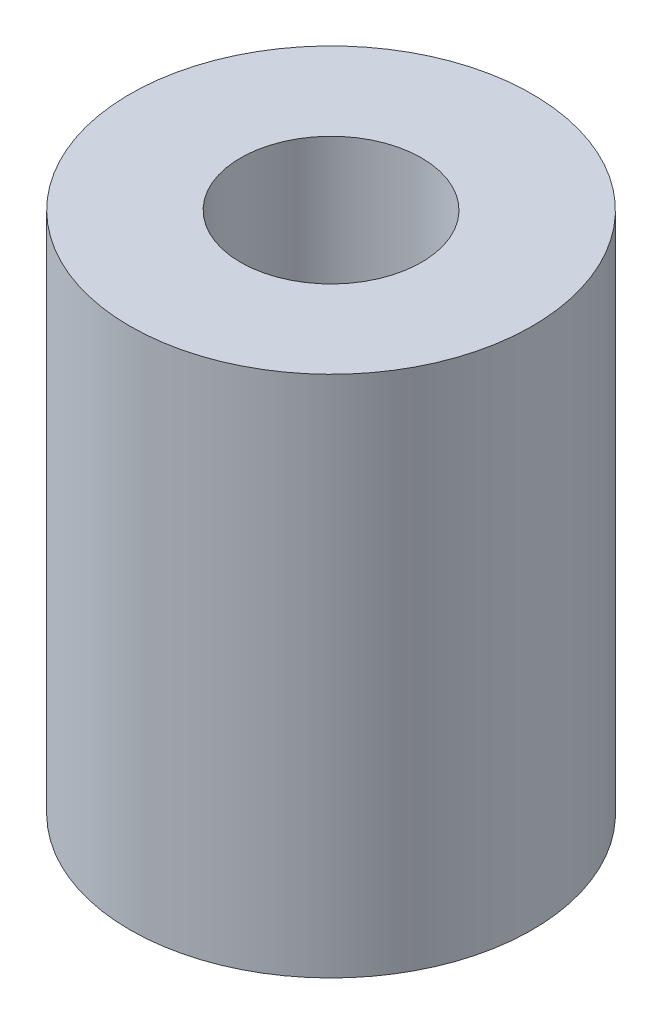
from build123d import *

# Parameters (mm, degrees)
SKETCH_1_R      = 50
SKETCH_1_R_2    = 22.5
EXTRUDE_1_DEPTH = 130


with BuildPart() as part:
    # 草图1 → 凸台-拉伸1 (new body)
    with BuildSketch(Plane(origin=(0, 0, 0), x_dir=(1, 0, 0), z_dir=(0, 1, 0))):
        with Locations(Location((0, 0, 0), (0, 0, 270))):
            Circle(SKETCH_1_R)
        with Locations(Location((0, 0, 0), (0, 0, 270))):
            Circle(SKETCH_1_R_2, mode=Mode.SUBTRACT)
    extrude(amount=EXTRUDE_1_DEPTH)


solid = part.part
